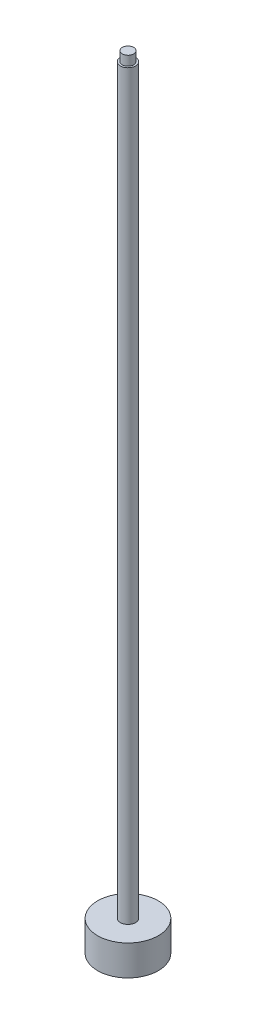
from build123d import *


with BuildPart() as part:
    # Sketch1 → Revolve1 (revolve)
    with BuildSketch(Plane.XY, mode=Mode.PRIVATE) as revolve1_sk:
        Polygon((0, 0), (30, 0), (30, 50), (160, 50), (160, 210), (40, 210), (40, 4126), (30, 4126), (30, 4176), (0, 4176), align=None)
    revolve(revolve1_sk.sketch.rotate(Axis((0, 4176, 0), (0, -1, 0)), 180), axis=Axis((0, 4176, 0), (0, -1, 0)))


solid = part.part
